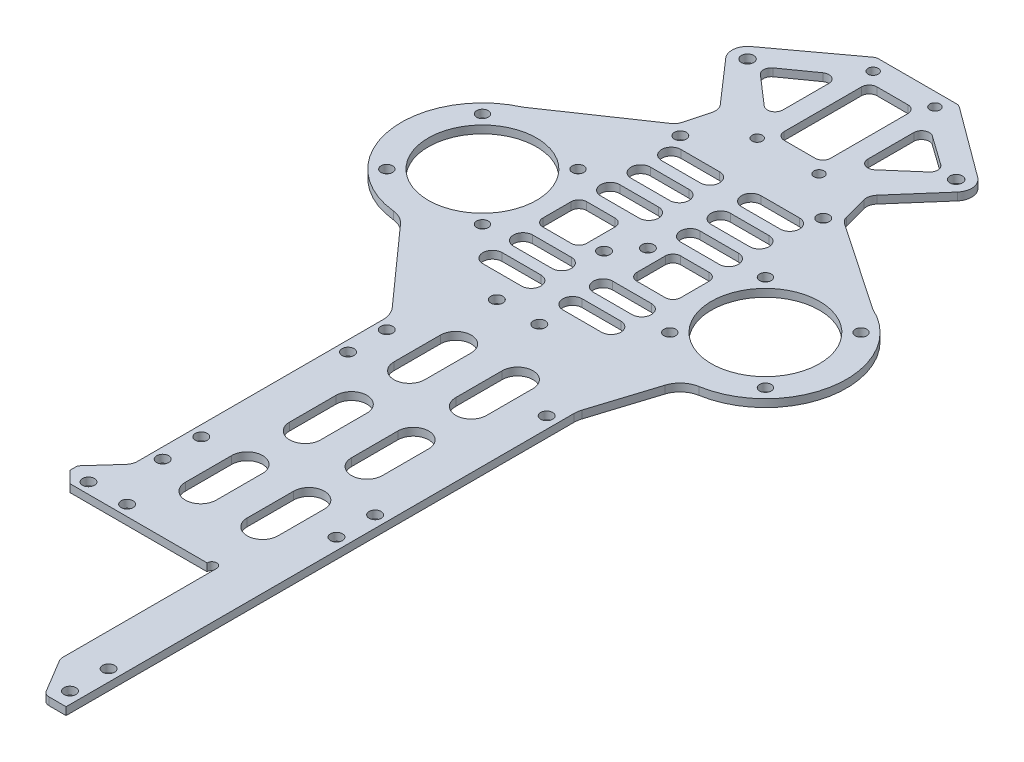
from build123d import *

# Parameters (mm, degrees)
SKETCH_1_R          = 14
SKETCH_1_R_2        = 1.5
SKETCH_1_R_3        = 1.325
SKETCH_1_R_4        = 1.55
EXTRUDE_1_DEPTH     = 2
SKETCH_2_R          = 1.6
EXTRUDE_2_DEPTH     = 2
SKETCH_3_R          = 1.25
SKETCH_3_W          = 12
SKETCH_3_H          = 24
SKETCH_3_W_2        = 11.35
SKETCH_3_H_2        = 11.35
CUT_EXTRUDE_1_DEPTH = 2
FILLET_1_R          = 2
FILLET_2_R          = 3
FILLET_3_R          = 6
CHAMFER_1_SIZE      = 3


with BuildPart() as part:
    # 草图1 → 凸台-拉伸1 (new body)
    with BuildSketch(Plane(origin=(0, 0, 0), x_dir=(1, 0, 0), z_dir=(0, 1, 0))):
        with BuildLine():
            Line((-10.689413765, 76), (10.689413765, 76))
            Line((10.689413765, 76), (21.546064807, 35.261709423))
            Line((21.546064807, 35.261709423), (45.279897923, 19.133550166))
            ThreePointArc((45.279897923, 19.133550166), (57.153085072, -4.426931585), (36.625, -21))
            Line((36.625, -21), (30, -42))
            Line((30, -42), (30, -105.4))
            Line((30, -105.4), (30, -174.4))
            Line((30, -174.4), (24.5, -174.4))
            Line((24.5, -174.4), (18.5, -164.4))
            Line((18.5, -164.4), (18.5, -123.9))
            Line((18.5, -123.9), (-22.5, -123.9))
            Line((-22.5, -123.9), (-22.5, -118.9))
            Line((-22.5, -118.9), (-15.75, -111.4))
            Line((-15.75, -111.4), (-15.75, -44.4))
            Line((-15.75, -44.4), (-36.625, -21))
            ThreePointArc((-36.625, -21), (-57.153085072, -4.426931585), (-45.279897923, 19.133550166))
            Line((-45.279897923, 19.133550166), (-21.546064807, 35.261709423))
            Line((-21.546064807, 35.261709423), (-10.689413765, 76))
        make_face()
        with Locations(Location((-36.625, 0, 0), (0, 0, 270))):
            Circle(SKETCH_1_R, mode=Mode.SUBTRACT)
        with Locations(Location((-24.250631329, 12.374368671, 0), (0, 0, 270))):
            Circle(SKETCH_1_R_2, mode=Mode.SUBTRACT)
        with Locations(Location((-24.250631329, -12.374368671, 0), (0, 0, 270))):
            Circle(SKETCH_1_R_2, mode=Mode.SUBTRACT)
        with Locations(Location((-48.999368671, -12.374368671, 0), (0, 0, 270))):
            Circle(SKETCH_1_R_2, mode=Mode.SUBTRACT)
        with Locations(Location((-48.999368671, 12.374368671, 0), (0, 0, 270))):
            Circle(SKETCH_1_R_2, mode=Mode.SUBTRACT)
        with Locations(Location((-8, 42.5, 0), (0, 0, 270))):
            Circle(SKETCH_1_R_3, mode=Mode.SUBTRACT)
        with Locations(Location((-8, 72.5, 0), (0, 0, 270))):
            Circle(SKETCH_1_R_3, mode=Mode.SUBTRACT)
        with Locations(Location((8, 42.5, 0), (0, 0, 90))):
            Circle(SKETCH_1_R_3, mode=Mode.SUBTRACT)
        with Locations(Location((8, 72.5, 0), (0, 0, 90))):
            Circle(SKETCH_1_R_3, mode=Mode.SUBTRACT)
        with Locations(Location((-18.5, 33.1, 0), (0, 0, 270))):
            Circle(SKETCH_1_R_4, mode=Mode.SUBTRACT)
        with Locations(Location((18.5, 33.1, 0), (0, 0, 90))):
            Circle(SKETCH_1_R_4, mode=Mode.SUBTRACT)
        with Locations(Location((24.250631329, -12.374368671, 0), (0, 0, 90))):
            Circle(SKETCH_1_R_2, mode=Mode.SUBTRACT)
        with Locations(Location((24.250631329, 12.374368671, 0), (0, 0, 90))):
            Circle(SKETCH_1_R_2, mode=Mode.SUBTRACT)
        with Locations(Location((48.999368671, 12.374368671, 0), (0, 0, 90))):
            Circle(SKETCH_1_R_2, mode=Mode.SUBTRACT)
        with Locations(Location((48.999368671, -12.374368671, 0), (0, 0, 90))):
            Circle(SKETCH_1_R_2, mode=Mode.SUBTRACT)
        with Locations(Location((36.625, 0, 0), (0, 0, 90))):
            Circle(SKETCH_1_R, mode=Mode.SUBTRACT)
        with Locations(Location((-5.5, -27.4, 0), (0, 0, 270))):
            Circle(SKETCH_1_R_4, mode=Mode.SUBTRACT)
        with Locations(Location((5.5, -27.4, 0), (0, 0, 90))):
            Circle(SKETCH_1_R_4, mode=Mode.SUBTRACT)
        with Locations(Location((27, -47, 0), (0, 0, 270))):
            Circle(SKETCH_1_R_4, mode=Mode.SUBTRACT)
        with Locations(Location((-13, -48.4, 0), (0, 0, 270))):
            Circle(SKETCH_1_R_4, mode=Mode.SUBTRACT)
        with Locations(Location((-13, -58.4, 0), (0, 0, 270))):
            Circle(SKETCH_1_R_4, mode=Mode.SUBTRACT)
        with Locations(Location((-13, -96.4, 0), (0, 0, 270))):
            Circle(SKETCH_1_R_4, mode=Mode.SUBTRACT)
        with Locations(Location((-13, -106.4, 0), (0, 0, 270))):
            Circle(SKETCH_1_R_4, mode=Mode.SUBTRACT)
        with Locations(Location((27, -91.4, 0), (0, 0, 270))):
            Circle(SKETCH_1_R_4, mode=Mode.SUBTRACT)
        with Locations(Location((27, -101.4, 0), (0, 0, 270))):
            Circle(SKETCH_1_R_4, mode=Mode.SUBTRACT)
        with Locations(Location((-7.5, -121.1, 0), (0, 0, 270))):
            Circle(SKETCH_1_R_4, mode=Mode.SUBTRACT)
        with Locations(Location((-17.5, -121.1, 0), (0, 0, 270))):
            Circle(SKETCH_1_R_4, mode=Mode.SUBTRACT)
        with Locations(Location((27, -170.4, 0), (0, 0, 270))):
            Circle(SKETCH_1_R_4, mode=Mode.SUBTRACT)
        with Locations(Location((27, -160.4, 0), (0, 0, 270))):
            Circle(SKETCH_1_R_4, mode=Mode.SUBTRACT)
        with Locations(Location((2.5, 3.7, 0), (0, 0, 270))):
            Circle(SKETCH_1_R_4, mode=Mode.SUBTRACT)
        with Locations(Location((-2.5, -2.65, 0), (0, 0, 270))):
            Circle(SKETCH_1_R_4, mode=Mode.SUBTRACT)
    extrude(amount=EXTRUDE_1_DEPTH)

    # 草图2 → 凸台-拉伸2 (add)
    # profile 1 of 2: a face of its own
    with BuildSketch(Plane(origin=(0, 2, 0), x_dir=(1, 0, 0), z_dir=(0, 1, 0))):
        with BuildLine():
            Line((10.689413765, 76), (19.217332547, 44))
            Line((19.217332547, 44), (30.013596127, 56.369745567))
            ThreePointArc((30.013596127, 56.369745567), (30.976318937, 59.434612141), (29.37425581, 62.219147302))
            Line((29.37425581, 62.219147302), (10.689413765, 76))
        make_face()
        with Locations(Location((27, 59, 0), (0, 0, 270))):
            Circle(SKETCH_2_R, mode=Mode.SUBTRACT)
    # profile 2 of 2: a face of its own
    with BuildSketch(Plane(origin=(0, 2, 0), x_dir=(1, 0, 0), z_dir=(0, 1, 0))):
        with BuildLine():
            Line((-19.217332547, 44), (-30.013596127, 56.369745567))
            ThreePointArc((-30.013596127, 56.369745567), (-30.976318937, 59.434612141), (-29.37425581, 62.219147302))
            Line((-29.37425581, 62.219147302), (-10.689413765, 76))
            Line((-10.689413765, 76), (-19.217332547, 44))
        make_face()
        with Locations(Location((-27, 59, 0), (0, 0, 90))):
            Circle(SKETCH_2_R, mode=Mode.SUBTRACT)
    extrude(amount=-EXTRUDE_2_DEPTH)

    # 草图3 → 切除-拉伸1 (cut)
    with BuildSketch(Plane(origin=(0, 2, 0), x_dir=(1, 0, 0), z_dir=(0, 1, 0))):
        with Locations((17.25, -123.9)):
            Circle(SKETCH_3_R)
        with Locations((0, 57.5)):
            Rectangle(SKETCH_3_W, SKETCH_3_H)
        Polygon((11, 67.914976417), (11, 47.754153586), (23.768521126, 58.842606143), align=None)
        Polygon((-11, 47.754153586), (-23.768521126, 58.842606143), (-11, 67.914976417), align=None)
        with BuildLine():
            Line((-15.35, 22.2), (-5.35, 22.2))
            ThreePointArc((-5.35, 22.2), (-2.85, 19.7), (-5.35, 17.2))
            Line((-5.35, 17.2), (-15.35, 17.2))
            ThreePointArc((-15.35, 17.2), (-17.85, 19.7), (-15.35, 22.2))
        make_face()
        with BuildLine():
            Line((-15.35, 14.3), (-5.35, 14.3))
            ThreePointArc((-5.35, 14.3), (-2.85, 11.8), (-5.35, 9.3))
            Line((-5.35, 9.3), (-15.35, 9.3))
            ThreePointArc((-15.35, 9.3), (-17.85, 11.8), (-15.35, 14.3))
        make_face()
        with BuildLine():
            Line((-15.35, 30.1), (-5.35, 30.1))
            ThreePointArc((-5.35, 30.1), (-2.85, 27.6), (-5.35, 25.1))
            Line((-5.35, 25.1), (-15.35, 25.1))
            ThreePointArc((-15.35, 25.1), (-17.85, 27.6), (-15.35, 30.1))
        make_face()
        with Locations((-12.175, 0.525)):
            Rectangle(SKETCH_3_W_2, SKETCH_3_H_2)
        with BuildLine():
            Line((-15.35, -8.25), (-5.35, -8.25))
            ThreePointArc((-5.35, -8.25), (-2.85, -10.75), (-5.35, -13.25))
            Line((-5.35, -13.25), (-15.35, -13.25))
            ThreePointArc((-15.35, -13.25), (-17.85, -10.75), (-15.35, -8.25))
        make_face()
        with BuildLine():
            Line((-15.35, -16.15), (-5.35, -16.15))
            ThreePointArc((-5.35, -16.15), (-2.85, -18.65), (-5.35, -21.15))
            Line((-5.35, -21.15), (-15.35, -21.15))
            ThreePointArc((-15.35, -21.15), (-17.85, -18.65), (-15.35, -16.15))
        make_face()
        with BuildLine():
            Line((15.35, 30.1), (5.35, 30.1))
            ThreePointArc((5.35, 30.1), (2.85, 27.6), (5.35, 25.1))
            Line((5.35, 25.1), (15.35, 25.1))
            ThreePointArc((15.35, 25.1), (17.85, 27.6), (15.35, 30.1))
        make_face()
        with BuildLine():
            Line((15.35, 22.2), (5.35, 22.2))
            ThreePointArc((5.35, 22.2), (2.85, 19.7), (5.35, 17.2))
            Line((5.35, 17.2), (15.35, 17.2))
            ThreePointArc((15.35, 17.2), (17.85, 19.7), (15.35, 22.2))
        make_face()
        with BuildLine():
            Line((15.35, 14.3), (5.35, 14.3))
            ThreePointArc((5.35, 14.3), (2.85, 11.8), (5.35, 9.3))
            Line((5.35, 9.3), (15.35, 9.3))
            ThreePointArc((15.35, 9.3), (17.85, 11.8), (15.35, 14.3))
        make_face()
        with Locations((12.175, 0.525)):
            Rectangle(SKETCH_3_W_2, SKETCH_3_H_2)
        with BuildLine():
            Line((15.35, -8.25), (5.35, -8.25))
            ThreePointArc((5.35, -8.25), (2.85, -10.75), (5.35, -13.25))
            Line((5.35, -13.25), (15.35, -13.25))
            ThreePointArc((15.35, -13.25), (17.85, -10.75), (15.35, -8.25))
        make_face()
        with BuildLine():
            Line((15.35, -16.15), (5.35, -16.15))
            ThreePointArc((5.35, -16.15), (2.85, -18.65), (5.35, -21.15))
            Line((5.35, -21.15), (15.35, -21.15))
            ThreePointArc((15.35, -21.15), (17.85, -18.65), (15.35, -16.15))
        make_face()
        with BuildLine():
            Line((3.125, -42.65), (3.125, -54.65))
            ThreePointArc((3.125, -54.65), (-0.875, -58.65), (-4.875, -54.65))
            Line((-4.875, -54.65), (-4.875, -42.65))
            ThreePointArc((-4.875, -42.65), (-0.875, -38.65), (3.125, -42.65))
        make_face()
        with BuildLine():
            Line((3.125, -69.65), (3.125, -81.65))
            ThreePointArc((3.125, -81.65), (-0.875, -85.65), (-4.875, -81.65))
            Line((-4.875, -81.65), (-4.875, -69.65))
            ThreePointArc((-4.875, -69.65), (-0.875, -65.65), (3.125, -69.65))
        make_face()
        with BuildLine():
            Line((3.125, -96.65), (3.125, -108.65))
            ThreePointArc((3.125, -108.65), (-0.875, -112.65), (-4.875, -108.65))
            Line((-4.875, -108.65), (-4.875, -96.65))
            ThreePointArc((-4.875, -96.65), (-0.875, -92.65), (3.125, -96.65))
        make_face()
        with BuildLine():
            Line((11.125, -96.65), (11.125, -108.65))
            ThreePointArc((11.125, -108.65), (15.125, -112.65), (19.125, -108.65))
            Line((19.125, -108.65), (19.125, -96.65))
            ThreePointArc((19.125, -96.65), (15.125, -92.65), (11.125, -96.65))
        make_face()
        with BuildLine():
            Line((11.125, -69.65), (11.125, -81.65))
            ThreePointArc((11.125, -81.65), (15.125, -85.65), (19.125, -81.65))
            Line((19.125, -81.65), (19.125, -69.65))
            ThreePointArc((19.125, -69.65), (15.125, -65.65), (11.125, -69.65))
        make_face()
        with BuildLine():
            Line((11.125, -42.65), (11.125, -54.65))
            ThreePointArc((11.125, -54.65), (15.125, -58.65), (19.125, -54.65))
            Line((19.125, -54.65), (19.125, -42.65))
            ThreePointArc((19.125, -42.65), (15.125, -38.65), (11.125, -42.65))
        make_face()
    extrude(amount=-CUT_EXTRUDE_1_DEPTH, mode=Mode.SUBTRACT)

    # 圆角1
    fillet_1_edges = [part.edges().sort_by_distance(p)[0] for p in [
        (-10.689413765, 1, -76),
        (10.689413765, 1, -76),
        (24.5, 1, 174.4),
        (18.5, 1, 164.4),
        (-17.85, 1, 5.15),
        (-17.85, 1, -6.2),
        (-6.5, 1, -6.2),
        (-6.5, 1, 5.15),
        (6, 1, -69.5),
        (6, 1, -45.5),
        (-6, 1, -45.5),
        (-6, 1, -69.5),
        (11, 1, -67.914976417),
        (23.768521126, 1, -58.842606143),
        (11, 1, -47.754153586),
        (-11, 1, -67.914976417),
        (-11, 1, -47.754153586),
        (-23.768521126, 1, -58.842606143),
        (17.85, 1, -6.2),
        (17.85, 1, 5.15),
        (6.5, 1, 5.15),
        (6.5, 1, -6.2),
    ]]
    fillet(fillet_1_edges, radius=FILLET_1_R)

    # 圆角2
    fillet_2_edges = [part.edges().sort_by_distance(p)[0] for p in [
        (19.217332547, 1, -44),
        (-19.217332547, 1, -44),
        (21.546064807, 1, -35.261709423),
        (-15.75, 1, 111.4),
        (-21.546064807, 1, -35.261709423),
    ]]
    fillet(fillet_2_edges, radius=FILLET_2_R)

    # 圆角3
    fillet_3_edges = [part.edges().sort_by_distance(p)[0] for p in [
        (36.625, 1, 21),
        (30, 1, 42),
        (-15.75, 1, 44.4),
        (-36.625, 1, 21),
    ]]
    fillet(fillet_3_edges, radius=FILLET_3_R)

    # 倒角1
    chamfer_1_edges = [part.edges().sort_by_distance(p)[0] for p in [
        (-22.5, 1, 123.9),
    ]]
    chamfer(chamfer_1_edges, length=CHAMFER_1_SIZE)


solid = part.part
